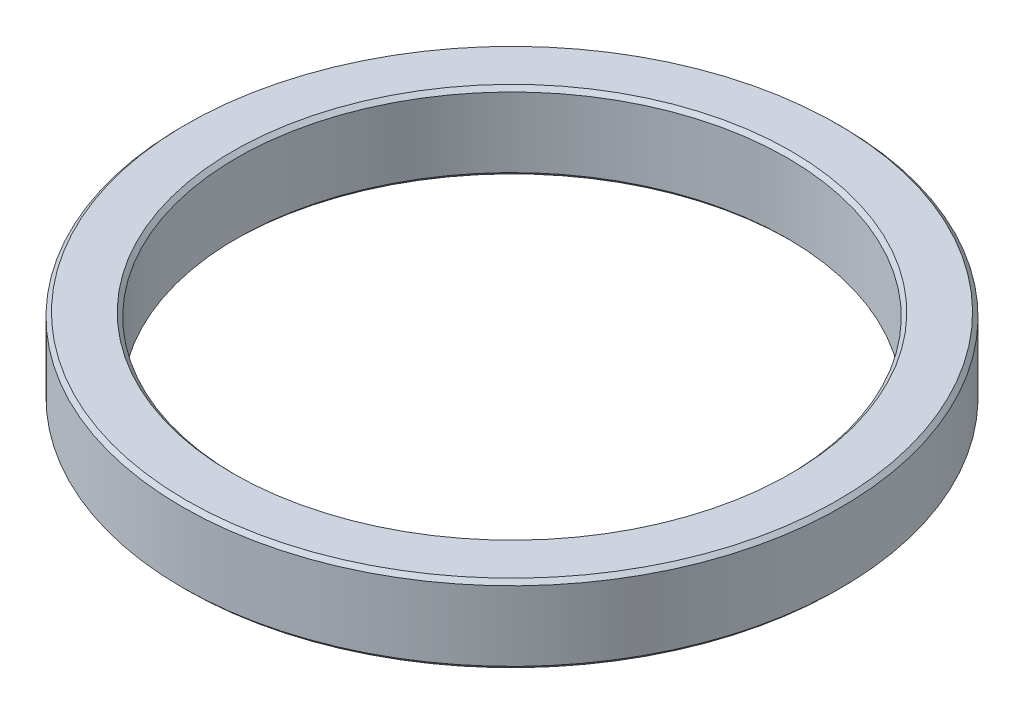
from build123d import *

# Parameters (mm, degrees)
SKETCH1_R           = 42.5
SKETCH1_R_2         = 35.5
BOSS_EXTRUDE1_DEPTH = 10
CHAMFER2_SIZE       = 0.5


with BuildPart() as part:
    # Sketch1 → Boss-Extrude1 (new body)
    with BuildSketch(Plane(origin=(0, 0, 0), x_dir=(1, 0, 0), z_dir=(0, 1, 0))):
        with Locations(Location((0, 0, 0), (0, 0, 270))):
            Circle(SKETCH1_R)
        with Locations(Location((0, 0, 0), (0, 0, 270))):
            Circle(SKETCH1_R_2, mode=Mode.SUBTRACT)
    extrude(amount=BOSS_EXTRUDE1_DEPTH)

    # Chamfer2
    chamfer2_edges = [part.edges().sort_by_distance(p)[0] for p in [
        (0, 0, -42.5),
        (0, 10, -42.5),
        (0, 0, -35.5),
        (0, 10, -35.5),
    ]]
    chamfer(chamfer2_edges, length=CHAMFER2_SIZE)


solid = part.part
